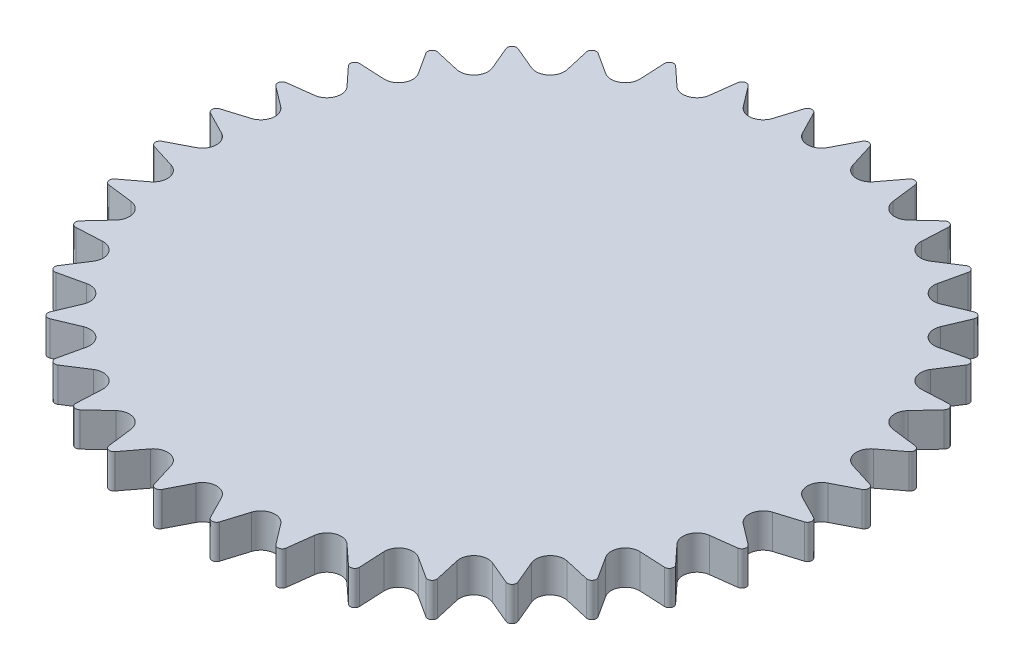
SolidWorks part; units mm, degrees
ref_plane "Front Plane" through (0, 0, 0) normal (0, 0, 1) x (1, 0, 0)
ref_plane "Top Plane" through (0, 0, 0) normal (0, 1, 0) x (1, 0, 0)
ref_plane "Right Plane" through (0, 0, 0) normal (1, 0, 0) x (0, 0, -1)
sketch "草图1" plane through (0, 0, 0) normal (0, 1, 0) x (1, 0, 0)
  circle A0 centre (0, 0) radius 290
  dimension "D1" = 580
extrude "Boss-Extrude1" add sketch "草图1" along normal blind 30
sketch "草图2" plane through (0, 30, 0) normal (0, 1, 0) x (1, 0, 0)
  line L0 (0, 290) -> (0, -290) construction
  circle A0 centre (0, 0) radius 290 construction
  circle A1 centre (-30, 160) radius 12.5
  circle A2 centre (30, 160) radius 12.5
  circle A3 centre (-100, -185) radius 15
  circle A4 centre (100, -185) radius 15
  dimension "D1" = 25
  dimension "D2" = 25
  dimension "D7" = 30
  dimension "D8" = 30
  dimension "D3" = 30
  dimension "D4" = 30
  dimension "D5" = 160
  dimension "D6" = 160
  dimension "D9" = 100
  dimension "D10" = 100
  dimension "D11" = 185
  dimension "D12" = 185
extrude "Boss-Extrude2" [suppressed] add sketch "草图2" along normal blind 85
ref_plane "Plane4" through (0, 15, 0) normal (0, 1, 0) x (1, 0, 0)
sketch "草图4" plane through (0, 30, 0) normal (0, 1, 0) x (1, 0, 0)
  line L0 (0, 272.5) -> (0, 0) construction
  line L1 (-25.2752, 288.8965) -> (0, 0) construction
  line L2 (0, 0) -> (25.2752, 288.8965) construction
  line L3 (-21.3686, 286.7396) -> (-11.1185, 266.7879)
  line L4 (11.1185, 266.7879) -> (21.3686, 286.7396)
  line L5 (57.2769, 260.8041) -> (70.8358, 278.6727)
  line L6 (28.7478, 286.094) -> (35.3776, 264.6655)
  line L7 (101.6948, 246.8959) -> (118.1506, 262.1385)
  line L8 (77.9908, 276.7555) -> (80.7988, 254.5014)
  line L9 (143.0229, 225.4858) -> (161.8755, 237.6394)
  line L10 (124.864, 259.008) -> (123.765, 236.6044)
  line L11 (180.0053, 197.2245) -> (200.6819, 205.9198)
  line L12 (167.9433, 233.3907) -> (162.9707, 211.5182)
  line L13 (211.5182, 162.9707) -> (233.3907, 167.9433)
  line L14 (205.9198, 200.6819) -> (197.2245, 180.0053)
  line L15 (236.6044, 123.765) -> (259.008, 124.864)
  line L16 (237.6394, 161.8755) -> (225.4858, 143.0229)
  line L17 (254.5014, 80.7988) -> (276.7555, 77.9908)
  line L18 (262.1385, 118.1506) -> (246.8959, 101.6948)
  line L19 (264.6655, 35.3776) -> (286.094, 28.7478)
  line L20 (278.6727, 70.8358) -> (260.8041, 57.2769)
  line L21 (266.7879, -11.1185) -> (286.7396, -21.3686)
  line L22 (286.7396, 21.3686) -> (266.7879, 11.1185)
  line L23 (260.8041, -57.2769) -> (278.6727, -70.8358)
  line L24 (286.094, -28.7478) -> (264.6655, -35.3776)
  line L25 (246.8959, -101.6948) -> (262.1385, -118.1506)
  line L26 (276.7555, -77.9908) -> (254.5014, -80.7988)
  line L27 (225.4858, -143.0229) -> (237.6394, -161.8755)
  line L28 (259.008, -124.864) -> (236.6044, -123.765)
  line L29 (197.2245, -180.0053) -> (205.9198, -200.6819)
  line L30 (233.3907, -167.9433) -> (211.5182, -162.9707)
  line L31 (162.9707, -211.5182) -> (167.9433, -233.3907)
  line L32 (200.6819, -205.9198) -> (180.0053, -197.2245)
  line L33 (123.765, -236.6044) -> (124.864, -259.008)
  line L34 (161.8755, -237.6394) -> (143.0229, -225.4858)
  line L35 (80.7988, -254.5014) -> (77.9908, -276.7555)
  line L36 (118.1506, -262.1385) -> (101.6948, -246.8959)
  line L37 (35.3776, -264.6655) -> (28.7478, -286.094)
  line L38 (70.8358, -278.6727) -> (57.2769, -260.8041)
  line L39 (-11.1185, -266.7879) -> (-21.3686, -286.7396)
  line L40 (21.3686, -286.7396) -> (11.1185, -266.7879)
  line L41 (-57.2769, -260.8041) -> (-70.8358, -278.6727)
  line L42 (-28.7478, -286.094) -> (-35.3776, -264.6655)
  line L43 (-101.6948, -246.8959) -> (-118.1506, -262.1385)
  line L44 (-77.9908, -276.7555) -> (-80.7988, -254.5014)
  line L45 (-143.0229, -225.4858) -> (-161.8755, -237.6394)
  line L46 (-124.864, -259.008) -> (-123.765, -236.6044)
  line L47 (-180.0053, -197.2245) -> (-200.6819, -205.9198)
  line L48 (-167.9433, -233.3907) -> (-162.9707, -211.5182)
  line L49 (-211.5182, -162.9707) -> (-233.3907, -167.9433)
  line L50 (-205.9198, -200.6819) -> (-197.2245, -180.0053)
  line L51 (-236.6044, -123.765) -> (-259.008, -124.864)
  line L52 (-237.6394, -161.8755) -> (-225.4858, -143.0229)
  line L53 (-254.5014, -80.7988) -> (-276.7555, -77.9908)
  line L54 (-262.1385, -118.1506) -> (-246.8959, -101.6948)
  line L55 (-264.6655, -35.3776) -> (-286.094, -28.7478)
  line L56 (-278.6727, -70.8358) -> (-260.8041, -57.2769)
  line L57 (-266.7879, 11.1185) -> (-286.7396, 21.3686)
  line L58 (-286.7396, -21.3686) -> (-266.7879, -11.1185)
  line L59 (-260.8041, 57.2769) -> (-278.6727, 70.8358)
  line L60 (-286.094, 28.7478) -> (-264.6655, 35.3776)
  line L61 (-246.8959, 101.6948) -> (-262.1385, 118.1506)
  line L62 (-276.7555, 77.9908) -> (-254.5014, 80.7988)
  line L63 (-225.4858, 143.0229) -> (-237.6394, 161.8755)
  line L64 (-259.008, 124.864) -> (-236.6044, 123.765)
  line L65 (-197.2245, 180.0053) -> (-205.9198, 200.6819)
  line L66 (-233.3907, 167.9433) -> (-211.5182, 162.9707)
  line L67 (-162.9707, 211.5182) -> (-167.9433, 233.3907)
  line L68 (-200.6819, 205.9198) -> (-180.0053, 197.2245)
  line L69 (-123.765, 236.6044) -> (-124.864, 259.008)
  line L70 (-161.8755, 237.6394) -> (-143.0229, 225.4858)
  line L71 (-80.7988, 254.5014) -> (-77.9908, 276.7555)
  line L72 (-118.1506, 262.1385) -> (-101.6948, 246.8959)
  line L73 (-35.3776, 264.6655) -> (-28.7478, 286.094)
  line L74 (-70.8358, 278.6727) -> (-57.2769, 260.8041)
  circle A0 centre (0, 0) radius 260 construction
  arc A1 (-11.1185, 266.7879) -> (11.1185, 266.7879) centre (0, 272.5) ccw
  circle A2 centre (0, 0) radius 290 construction
  arc A3 (-21.3686, 286.7396) -> (-25.2752, 288.8965) centre (-24.9265, 284.9117) ccw
  arc A4 (25.2752, 288.8965) -> (21.3686, 286.7396) centre (24.9265, 284.9117) ccw
  arc A6 (28.7478, 286.094) -> (25.2752, 288.8965) centre (24.9265, 284.9117) ccw
  arc A7 (75.0575, 280.1185) -> (70.8358, 278.6727) centre (74.0222, 276.2548) ccw
  arc A8 (35.3776, 264.6655) -> (57.2769, 260.8041) centre (47.3191, 268.3601) ccw
  arc A9 (77.9908, 276.7555) -> (75.0575, 280.1185) centre (74.0222, 276.2548) ccw
  arc A10 (122.5593, 262.8293) -> (118.1506, 262.1385) centre (120.8688, 259.204) ccw
  arc A11 (80.7988, 254.5014) -> (101.6948, 246.8959) centre (93.2005, 256.0662) ccw
  arc A12 (124.864, 259.008) -> (122.5593, 262.8293) centre (120.8688, 259.204) ccw
  arc A13 (166.3372, 237.5541) -> (161.8755, 237.6394) centre (164.0429, 234.2775) ccw
  arc A14 (123.765, 236.6044) -> (143.0229, 225.4858) centre (136.25, 235.9919) ccw
  arc A15 (167.9433, 233.3907) -> (166.3372, 237.5541) centre (164.0429, 234.2775) ccw
  arc A16 (205.061, 205.061) -> (200.6819, 205.9198) centre (202.2325, 202.2325) ccw
  arc A17 (162.9707, 211.5182) -> (180.0053, 197.2245) centre (175.1596, 208.7471) ccw
  arc A18 (205.9198, 200.6819) -> (205.061, 205.061) centre (202.2325, 202.2325) ccw
  arc A19 (237.5541, 166.3372) -> (233.3907, 167.9433) centre (234.2775, 164.0429) ccw
  arc A20 (197.2245, 180.0053) -> (211.5182, 162.9707) centre (208.7471, 175.1596) ccw
  arc A21 (237.6394, 161.8755) -> (237.5541, 166.3372) centre (234.2775, 164.0429) ccw
  arc A22 (262.8293, 122.5593) -> (259.008, 124.864) centre (259.204, 120.8688) ccw
  arc A23 (225.4858, 143.0229) -> (236.6044, 123.765) centre (235.9919, 136.25) ccw
  arc A24 (262.1385, 118.1506) -> (262.8293, 122.5593) centre (259.204, 120.8688) ccw
  arc A25 (280.1185, 75.0575) -> (276.7555, 77.9908) centre (276.2548, 74.0222) ccw
  arc A26 (246.8959, 101.6948) -> (254.5014, 80.7988) centre (256.0662, 93.2005) ccw
  arc A27 (278.6727, 70.8358) -> (280.1185, 75.0575) centre (276.2548, 74.0222) ccw
  arc A28 (288.8965, 25.2752) -> (286.094, 28.7478) centre (284.9117, 24.9265) ccw
  arc A29 (260.8041, 57.2769) -> (264.6655, 35.3776) centre (268.3601, 47.3191) ccw
  arc A30 (286.7396, 21.3686) -> (288.8965, 25.2752) centre (284.9117, 24.9265) ccw
  arc A31 (288.8965, -25.2752) -> (286.7396, -21.3686) centre (284.9117, -24.9265) ccw
  arc A32 (266.7879, 11.1185) -> (266.7879, -11.1185) centre (272.5, 0) ccw
  arc A33 (286.094, -28.7478) -> (288.8965, -25.2752) centre (284.9117, -24.9265) ccw
  arc A34 (280.1185, -75.0575) -> (278.6727, -70.8358) centre (276.2548, -74.0222) ccw
  arc A35 (264.6655, -35.3776) -> (260.8041, -57.2769) centre (268.3601, -47.3191) ccw
  arc A36 (276.7555, -77.9908) -> (280.1185, -75.0575) centre (276.2548, -74.0222) ccw
  arc A37 (262.8293, -122.5593) -> (262.1385, -118.1506) centre (259.204, -120.8688) ccw
  arc A38 (254.5014, -80.7988) -> (246.8959, -101.6948) centre (256.0662, -93.2005) ccw
  arc A39 (259.008, -124.864) -> (262.8293, -122.5593) centre (259.204, -120.8688) ccw
  arc A40 (237.5541, -166.3372) -> (237.6394, -161.8755) centre (234.2775, -164.0429) ccw
  arc A41 (236.6044, -123.765) -> (225.4858, -143.0229) centre (235.9919, -136.25) ccw
  arc A42 (233.3907, -167.9433) -> (237.5541, -166.3372) centre (234.2775, -164.0429) ccw
  arc A43 (205.061, -205.061) -> (205.9198, -200.6819) centre (202.2325, -202.2325) ccw
  arc A44 (211.5182, -162.9707) -> (197.2245, -180.0053) centre (208.7471, -175.1596) ccw
  arc A45 (200.6819, -205.9198) -> (205.061, -205.061) centre (202.2325, -202.2325) ccw
  arc A46 (166.3372, -237.5541) -> (167.9433, -233.3907) centre (164.0429, -234.2775) ccw
  arc A47 (180.0053, -197.2245) -> (162.9707, -211.5182) centre (175.1596, -208.7471) ccw
  arc A48 (161.8755, -237.6394) -> (166.3372, -237.5541) centre (164.0429, -234.2775) ccw
  arc A49 (122.5593, -262.8293) -> (124.864, -259.008) centre (120.8688, -259.204) ccw
  arc A50 (143.0229, -225.4858) -> (123.765, -236.6044) centre (136.25, -235.9919) ccw
  arc A51 (118.1506, -262.1385) -> (122.5593, -262.8293) centre (120.8688, -259.204) ccw
  arc A52 (75.0575, -280.1185) -> (77.9908, -276.7555) centre (74.0222, -276.2548) ccw
  arc A53 (101.6948, -246.8959) -> (80.7988, -254.5014) centre (93.2005, -256.0662) ccw
  arc A54 (70.8358, -278.6727) -> (75.0575, -280.1185) centre (74.0222, -276.2548) ccw
  arc A55 (25.2752, -288.8965) -> (28.7478, -286.094) centre (24.9265, -284.9117) ccw
  arc A56 (57.2769, -260.8041) -> (35.3776, -264.6655) centre (47.3191, -268.3601) ccw
  arc A57 (21.3686, -286.7396) -> (25.2752, -288.8965) centre (24.9265, -284.9117) ccw
  arc A58 (-25.2752, -288.8965) -> (-21.3686, -286.7396) centre (-24.9265, -284.9117) ccw
  arc A59 (11.1185, -266.7879) -> (-11.1185, -266.7879) centre (0, -272.5) ccw
  arc A60 (-28.7478, -286.094) -> (-25.2752, -288.8965) centre (-24.9265, -284.9117) ccw
  arc A61 (-75.0575, -280.1185) -> (-70.8358, -278.6727) centre (-74.0222, -276.2548) ccw
  arc A62 (-35.3776, -264.6655) -> (-57.2769, -260.8041) centre (-47.3191, -268.3601) ccw
  arc A63 (-77.9908, -276.7555) -> (-75.0575, -280.1185) centre (-74.0222, -276.2548) ccw
  arc A64 (-122.5593, -262.8293) -> (-118.1506, -262.1385) centre (-120.8688, -259.204) ccw
  arc A65 (-80.7988, -254.5014) -> (-101.6948, -246.8959) centre (-93.2005, -256.0662) ccw
  arc A66 (-124.864, -259.008) -> (-122.5593, -262.8293) centre (-120.8688, -259.204) ccw
  arc A67 (-166.3372, -237.5541) -> (-161.8755, -237.6394) centre (-164.0429, -234.2775) ccw
  arc A68 (-123.765, -236.6044) -> (-143.0229, -225.4858) centre (-136.25, -235.9919) ccw
  arc A69 (-167.9433, -233.3907) -> (-166.3372, -237.5541) centre (-164.0429, -234.2775) ccw
  arc A70 (-205.061, -205.061) -> (-200.6819, -205.9198) centre (-202.2325, -202.2325) ccw
  arc A71 (-162.9707, -211.5182) -> (-180.0053, -197.2245) centre (-175.1596, -208.7471) ccw
  arc A72 (-205.9198, -200.6819) -> (-205.061, -205.061) centre (-202.2325, -202.2325) ccw
  arc A73 (-237.5541, -166.3372) -> (-233.3907, -167.9433) centre (-234.2775, -164.0429) ccw
  arc A74 (-197.2245, -180.0053) -> (-211.5182, -162.9707) centre (-208.7471, -175.1596) ccw
  arc A75 (-237.6394, -161.8755) -> (-237.5541, -166.3372) centre (-234.2775, -164.0429) ccw
  arc A76 (-262.8293, -122.5593) -> (-259.008, -124.864) centre (-259.204, -120.8688) ccw
  arc A77 (-225.4858, -143.0229) -> (-236.6044, -123.765) centre (-235.9919, -136.25) ccw
  arc A78 (-262.1385, -118.1506) -> (-262.8293, -122.5593) centre (-259.204, -120.8688) ccw
  arc A79 (-280.1185, -75.0575) -> (-276.7555, -77.9908) centre (-276.2548, -74.0222) ccw
  arc A80 (-246.8959, -101.6948) -> (-254.5014, -80.7988) centre (-256.0662, -93.2005) ccw
  arc A81 (-278.6727, -70.8358) -> (-280.1185, -75.0575) centre (-276.2548, -74.0222) ccw
  arc A82 (-288.8965, -25.2752) -> (-286.094, -28.7478) centre (-284.9117, -24.9265) ccw
  arc A83 (-260.8041, -57.2769) -> (-264.6655, -35.3776) centre (-268.3601, -47.3191) ccw
  arc A84 (-286.7396, -21.3686) -> (-288.8965, -25.2752) centre (-284.9117, -24.9265) ccw
  arc A85 (-288.8965, 25.2752) -> (-286.7396, 21.3686) centre (-284.9117, 24.9265) ccw
  arc A86 (-266.7879, -11.1185) -> (-266.7879, 11.1185) centre (-272.5, 0) ccw
  arc A87 (-286.094, 28.7478) -> (-288.8965, 25.2752) centre (-284.9117, 24.9265) ccw
  arc A88 (-280.1185, 75.0575) -> (-278.6727, 70.8358) centre (-276.2548, 74.0222) ccw
  arc A89 (-264.6655, 35.3776) -> (-260.8041, 57.2769) centre (-268.3601, 47.3191) ccw
  arc A90 (-276.7555, 77.9908) -> (-280.1185, 75.0575) centre (-276.2548, 74.0222) ccw
  arc A91 (-262.8293, 122.5593) -> (-262.1385, 118.1506) centre (-259.204, 120.8688) ccw
  arc A92 (-254.5014, 80.7988) -> (-246.8959, 101.6948) centre (-256.0662, 93.2005) ccw
  arc A93 (-259.008, 124.864) -> (-262.8293, 122.5593) centre (-259.204, 120.8688) ccw
  arc A94 (-237.5541, 166.3372) -> (-237.6394, 161.8755) centre (-234.2775, 164.0429) ccw
  arc A95 (-236.6044, 123.765) -> (-225.4858, 143.0229) centre (-235.9919, 136.25) ccw
  arc A96 (-233.3907, 167.9433) -> (-237.5541, 166.3372) centre (-234.2775, 164.0429) ccw
  arc A97 (-205.061, 205.061) -> (-205.9198, 200.6819) centre (-202.2325, 202.2325) ccw
  arc A98 (-211.5182, 162.9707) -> (-197.2245, 180.0053) centre (-208.7471, 175.1596) ccw
  arc A99 (-200.6819, 205.9198) -> (-205.061, 205.061) centre (-202.2325, 202.2325) ccw
  arc A100 (-166.3372, 237.5541) -> (-167.9433, 233.3907) centre (-164.0429, 234.2775) ccw
  arc A101 (-180.0053, 197.2245) -> (-162.9707, 211.5182) centre (-175.1596, 208.7471) ccw
  arc A102 (-161.8755, 237.6394) -> (-166.3372, 237.5541) centre (-164.0429, 234.2775) ccw
  arc A103 (-122.5593, 262.8293) -> (-124.864, 259.008) centre (-120.8688, 259.204) ccw
  arc A104 (-143.0229, 225.4858) -> (-123.765, 236.6044) centre (-136.25, 235.9919) ccw
  arc A105 (-118.1506, 262.1385) -> (-122.5593, 262.8293) centre (-120.8688, 259.204) ccw
  arc A106 (-75.0575, 280.1185) -> (-77.9908, 276.7555) centre (-74.0222, 276.2548) ccw
  arc A107 (-101.6948, 246.8959) -> (-80.7988, 254.5014) centre (-93.2005, 256.0662) ccw
  arc A108 (-70.8358, 278.6727) -> (-75.0575, 280.1185) centre (-74.0222, 276.2548) ccw
  arc A109 (-25.2752, 288.8965) -> (-28.7478, 286.094) centre (-24.9265, 284.9117) ccw
  arc A110 (-57.2769, 260.8041) -> (-35.3776, 264.6655) centre (-47.3191, 268.3601) ccw
  circle A111 centre (0, 0) radius 330.9347
  point P331 (0, 0)
  dimension "D1" = 520
  dimension "D2" = 25
  dimension "D5" = 8
  dimension "D6" = 8
  dimension "D3" = 5
  dimension "D4" = 5
  dimension "D7" = 36
extrude "Cut-Extrude1" cut sketch "草图4" against normal blind 30
sketch "Sketch5" plane through (0, 30, 0) normal (0, 1, 0) x (1, 0, 0)
  circle A0 centre (0, 0) radius 260
  dimension "D1" = 520
